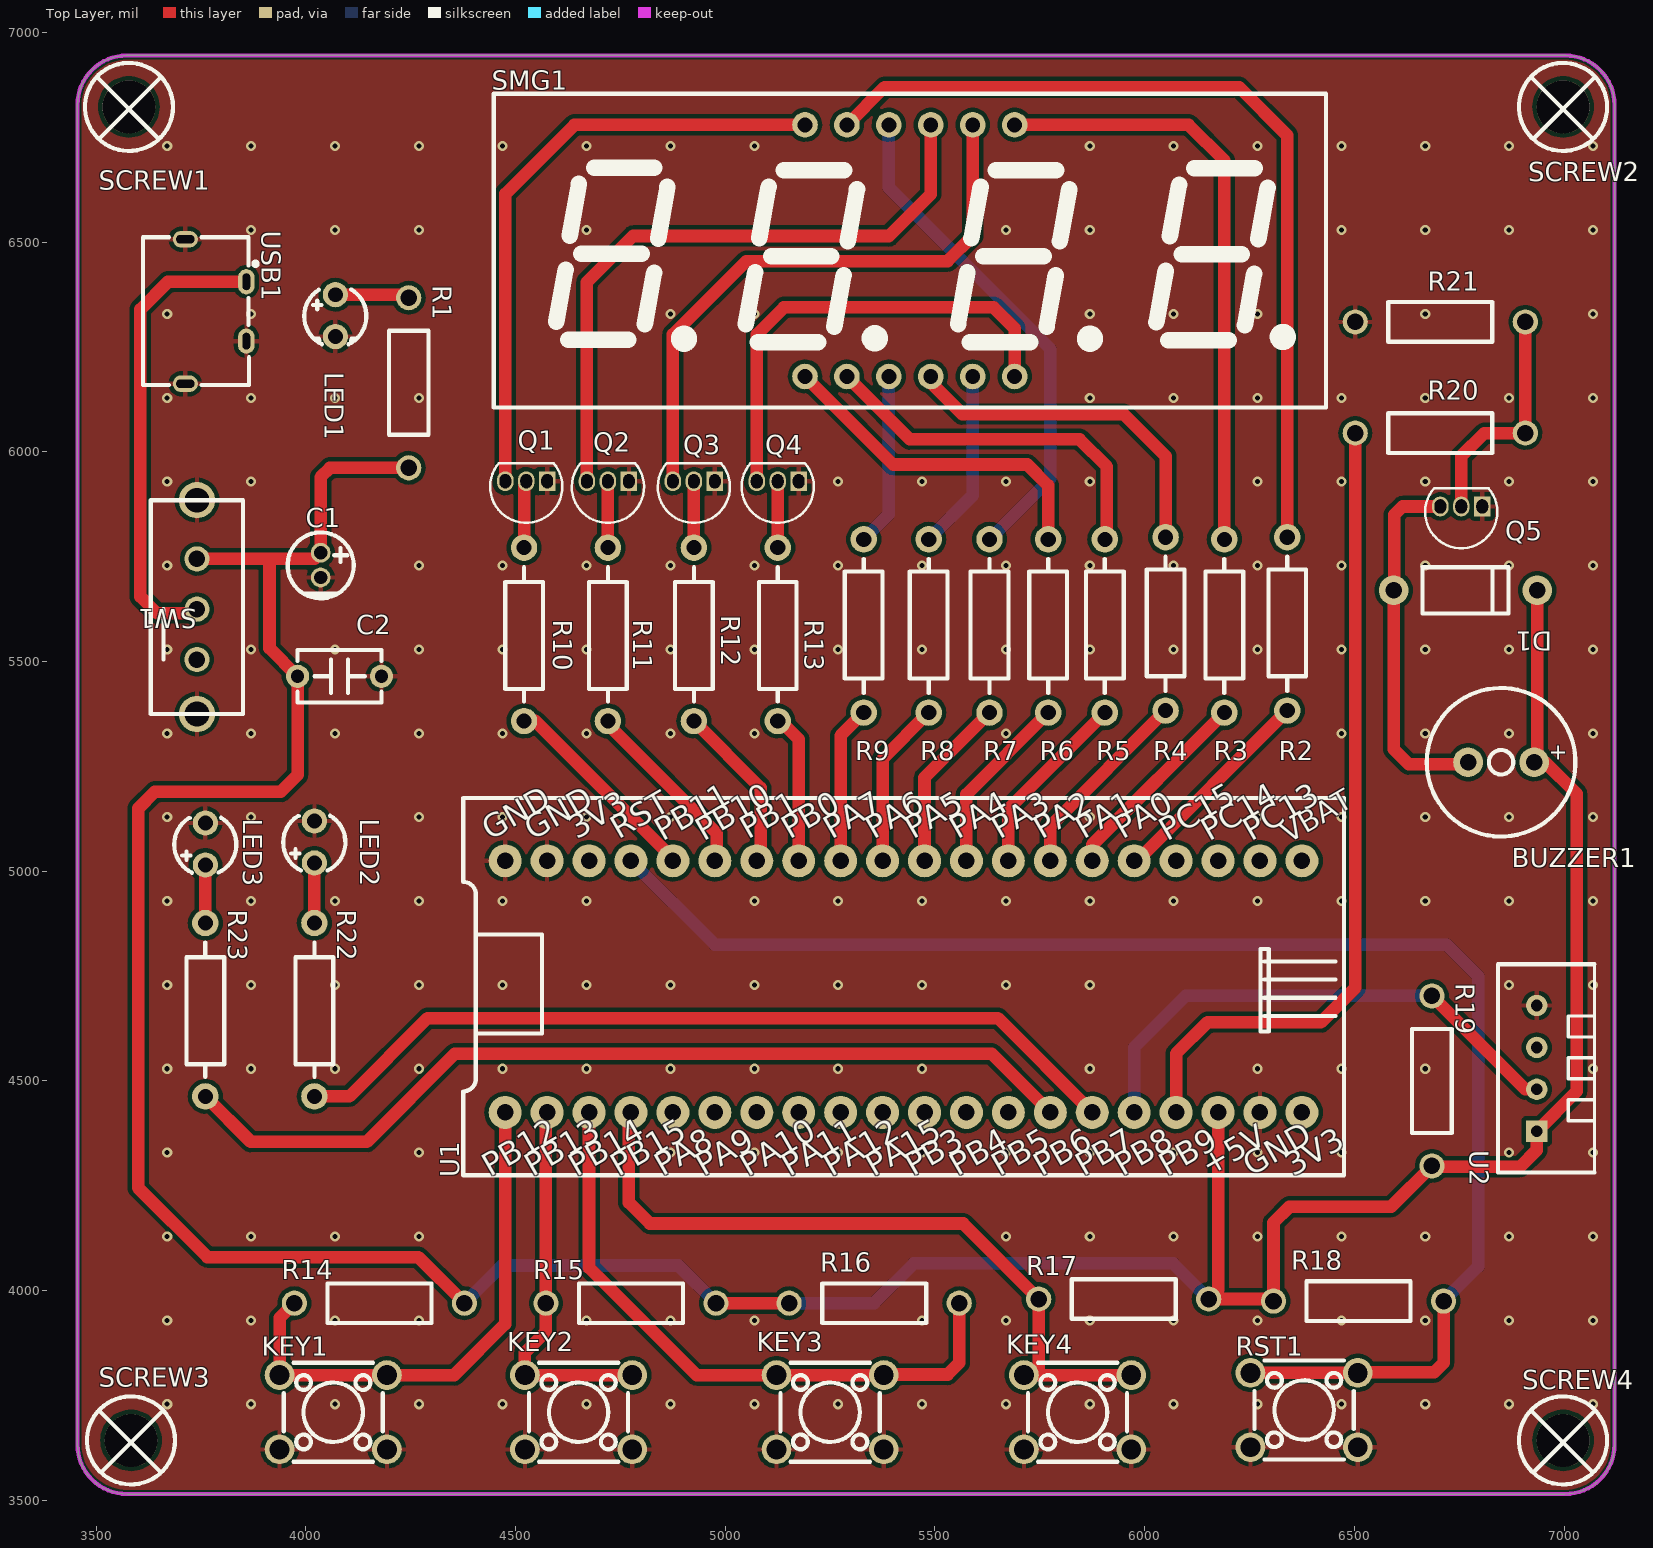
[diagram p0: Top Layer view]
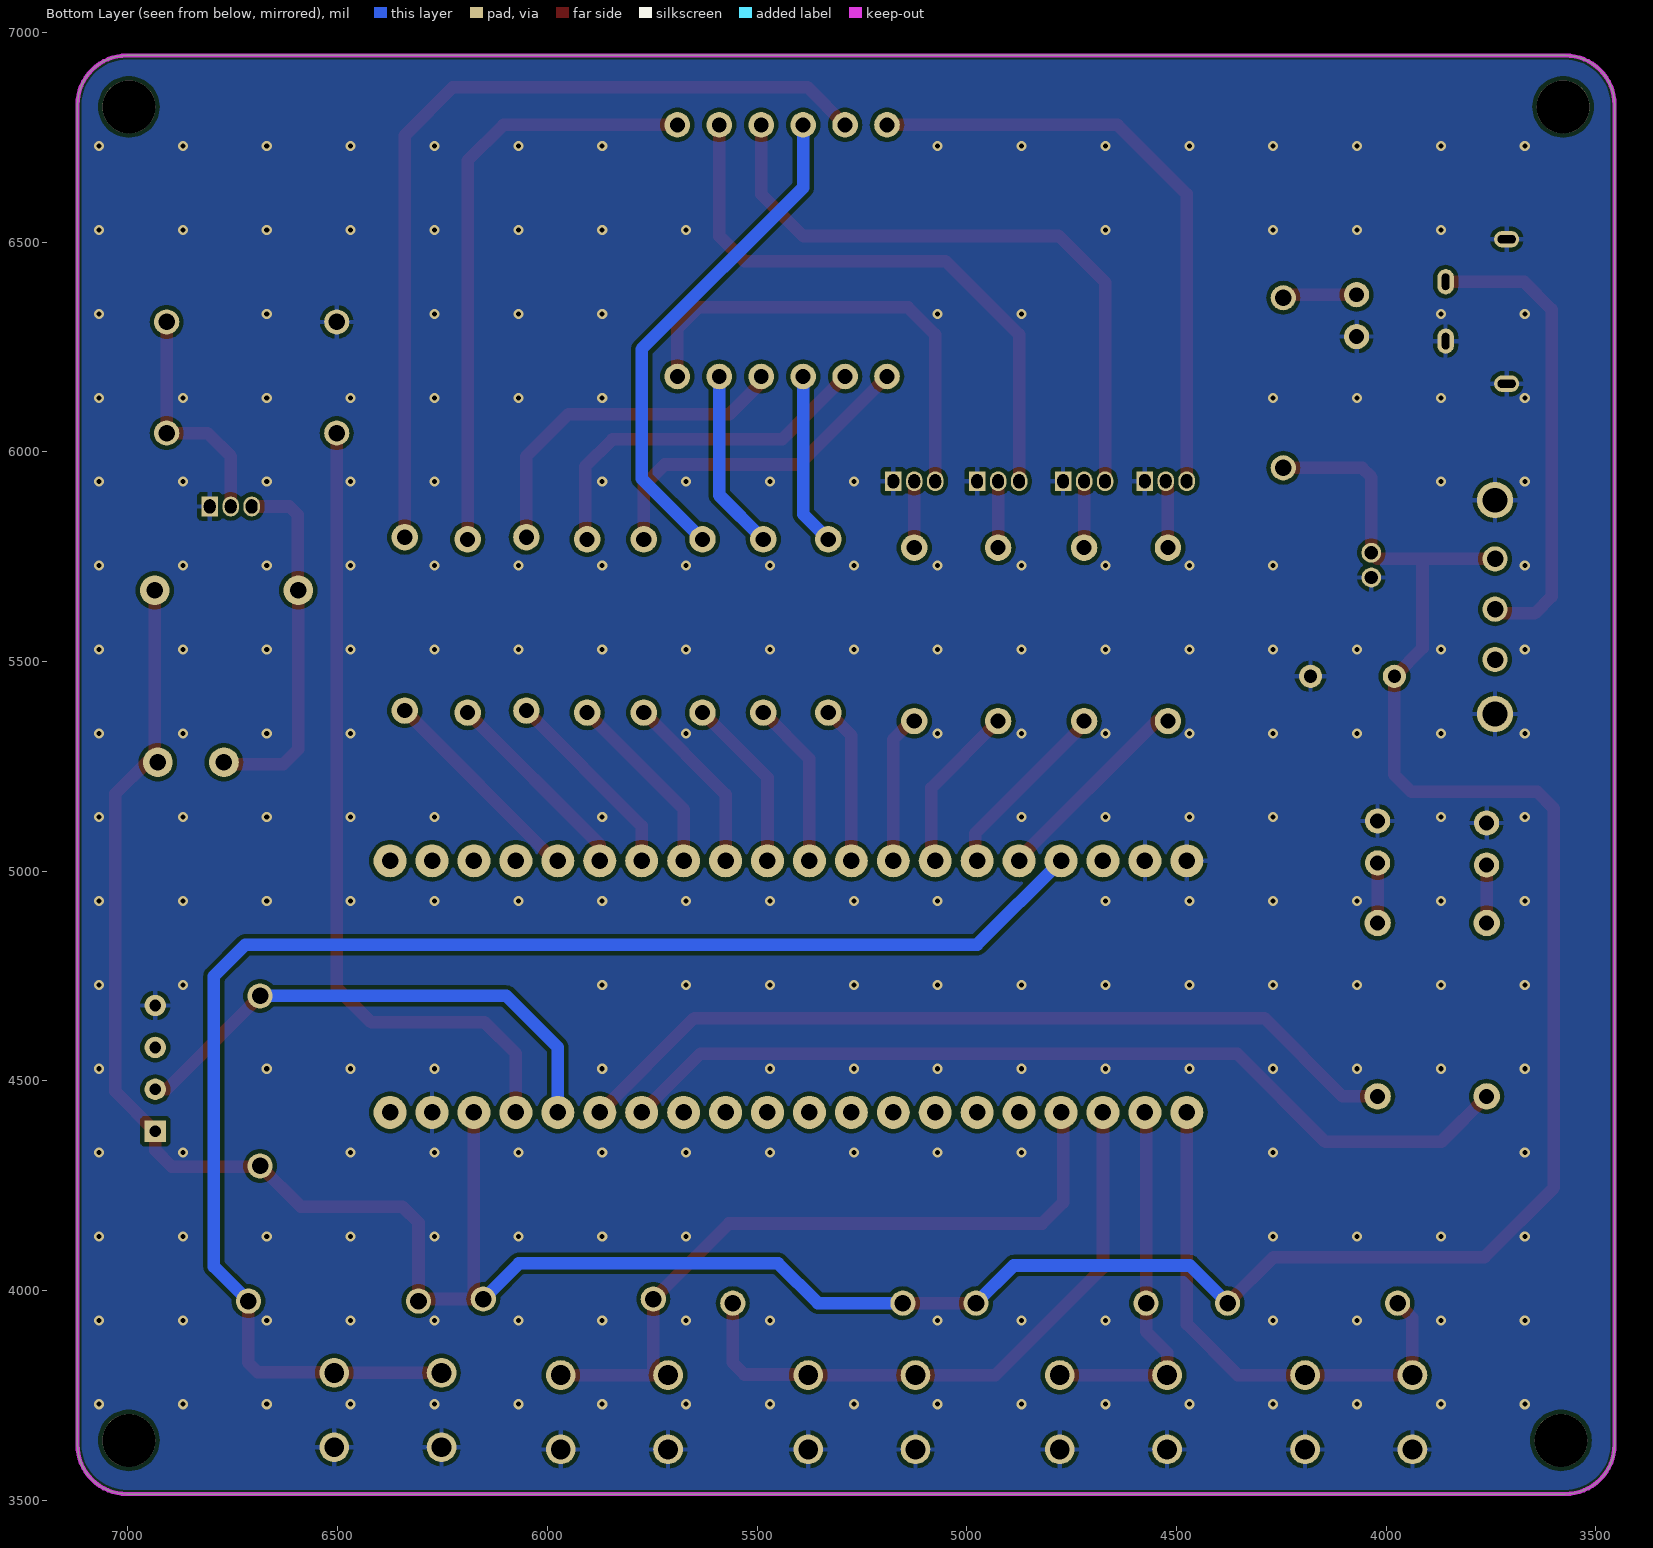
[diagram p1: Bottom Layer view, seen from below]
# Altium PCB MISC61551.pcbdoc
Units mil, origin at the board's own origin, x right, y up, seen from the top; angles counter-clockwise.
Board outline 3665.55 x 3430.55 mil, 2 copper layers (Top Layer, Bottom Layer), stack 62.206 mil thick; 49 components, 45 nets, 164 pads, 222 vias.

## Layer stack, top to bottom
Top Solder Mask Layer: solder mask 0.394, Dk 3.3
Top Layer: signal copper 1.379
Dielectric1: surface 59.449, FR4, Dk 4.5
Bottom Layer: signal copper 1.378
Bottom Solder Mask Layer: solder mask 0.394, Dk 3.3

## Board outline
3573.11,6945.55 ccw(c3573.11,6827.44) 3455,6827.44 3455,3633.11 ccw(c3573.11,3633.11) 3573.11,3515 7002.44,3515 ccw(c7002.44,3633.11) 7120.55,3633.11 7120.55,6827.44 ccw(c7002.44,6827.44) 7002.44,6945.55 3573.11,6945.55

## Design rules (kind name [scope] priority, off if disabled: settings)
BoardOutlineClearance copperThickness2oz_1 [All] p2 off: genericclearance=7.99 ignorepadtopadclearanceinfootprint=FALSE except(0: Arc-SplitContinuation Track-SplitContinuation SMDPad-SplitContinuation THPad-SplitContinuation Via-SplitContinuation Fill-SplitContinuation Region-SplitContinuation Poly-SplitContinuation Text-SplitContinuation Hole-SplitContinuation; 5.98: Arc-CutoutEdge SMDPad-CutoutEdge THPad-CutoutEdge Via-CutoutEdge Fill-CutoutEdge Region-CutoutEdge Text-CutoutEdge; 6.93: Hole-OutlineEdge Hole-CutoutEdge; 10: Poly-OutlineEdge Poly-CutoutEdge; 11.81: Arc-OutlineEdge Track-OutlineEdge SMDPad-OutlineEdge THPad-OutlineEdge Via-OutlineEdge Fill-OutlineEdge Region-OutlineEdge Text-OutlineEdge Track-CutoutEdge)
BoardOutlineClearance copperThickness1oz_1 [All] p4: genericclearance=6 ignorepadtopadclearanceinfootprint=FALSE except(0: Arc-SplitContinuation Track-SplitContinuation SMDPad-SplitContinuation THPad-SplitContinuation Via-SplitContinuation Fill-SplitContinuation Region-SplitContinuation Poly-SplitContinuation Text-SplitContinuation Hole-SplitContinuation; 6: SMDPad-CutoutEdge THPad-CutoutEdge Via-CutoutEdge Fill-CutoutEdge Region-CutoutEdge Text-CutoutEdge; 6.93: Hole-OutlineEdge Hole-CutoutEdge; 10: Poly-OutlineEdge Poly-CutoutEdge; 11.8: Arc-OutlineEdge Track-OutlineEdge SMDPad-OutlineEdge THPad-OutlineEdge Via-OutlineEdge Fill-OutlineEdge Region-OutlineEdge Text-OutlineEdge; 11.81: Arc-CutoutEdge Track-CutoutEdge)
Clearance copperThickness2oz [All] p1 off: gap=7.99 ignorepadtopadclearanceinfootprint=FALSE except(5.98: SMDPad-Track SMDPad-SMDPad THPad-Track SMDPad-THPad THPad-THPad Track-Via SMDPad-Via THPad-Via Via-Via Fill-Track Region-Track Fill-SMDPad Region-SMDPad Fill-THPad Region-THPad Fill-Via Region-Via Fill-Fill Fill-Region Region-Region Arc-Track Arc-SMDPad Arc-THPad Arc-Via Fill-Arc Region-Arc Arc-Arc Text-Track SMDPad-Text Text-THPad Text-Via Fill-Text Region-Text Arc-Text Text-Text; 6.93: Hole-Track Hole-SMDPad Hole-THPad Hole-Via Fill-Hole Region-Hole Hole-Arc Hole-Text; 10: Poly-Track Poly-SMDPad Poly-THPad Poly-Via Poly-Fill Poly-Region Poly-Poly Poly-Arc Poly-Text Poly-Hole)
Clearance copperThickness1oz [All] p3: gap=6 ignorepadtopadclearanceinfootprint=FALSE except(5.98: SMDPad-Track SMDPad-SMDPad THPad-Track SMDPad-THPad THPad-THPad Track-Via SMDPad-Via THPad-Via Via-Via Fill-Track Region-Track Fill-SMDPad Region-SMDPad Fill-THPad Region-THPad Fill-Via Region-Via Fill-Fill Fill-Region Region-Region; 6.93: Hole-Track Hole-SMDPad Hole-THPad Hole-Via Fill-Hole Region-Hole Hole-Arc Hole-Text; 10: Poly-Track Poly-SMDPad Poly-THPad Poly-Via Poly-Fill Poly-Region Poly-Poly Poly-Arc Poly-Text Poly-Hole)
DiffPairsRouting differentialPair [All] p1: maxlimit=6 minlimit=6 mostfreqgap=6 toplayer_minwidth=5 toplayer_prefwidth=10 toplayer_maxwidth=100 toplayer_mingap=6 toplayer_prefgap=6 toplayer_maxgap=6 bottomlayer_minwidth=5 bottomlayer_prefwidth=10 bottomlayer_maxwidth=100 bottomlayer_mingap=6 bottomlayer_prefgap=6 bottomlayer_maxgap=6 maxuncoupledlength=10
HoleToHoleClearance otherClearance [All] p1: gap=11.81 allowstackedmicrovias=TRUE
Length netLength [All] p1: minlimit=0 maxlimit=0
MatchedLengths netLengthTolerance [All] p1: tolerance=1000
PasteMaskExpansion pasteMaskExpansion [All] p1: expansion=0
PlaneConnect innerPlane [All] p1: planeconnectstyle=Relief reliefexpansion=20 reliefentries=4 reliefconductorwidth=10 reliefairgap=10
PolygonConnect copperRegion [(InNet('GND'))] p1: connectstyle=Relief reliefconductorwidth=10 reliefentries=4 polygonreliefangle="90 Angle" airgapwidth=10 via.connectstyle=Relief via.reliefconductorwidth=10 via.reliefentries=4 via.polygonreliefangle="90 Angle" via.airgapwidth=10
RoutingVias viaSize [All] p1: holewidth=12.01 width=24.02 viastyle="Through Hole" minholewidth=12 minwidth=24 maxholewidth=248.03 maxwidth=393.7
SolderMaskExpansion solderMaskExpansion [IsVia] p1: expansion=-1000 istentingtop=TRUE
SolderMaskExpansion solderMaskExpansion [All] p2: expansion=2 istentingtop=FALSE
Width copperThickness2oz_2 [All] p1 off: maxlimit=100 minlimit=8 preferedwidth=10
Width PWR [(InNet('+5V') OR InNet('BUZZER') OR InNet('DIG1') OR InNet('DIG2') OR InNet('DIG3') OR InNet('DIG4') OR InNet('VCC'))] p2: maxlimit=10 minlimit=10 preferedwidth=10 toplayer_minwidth=10 toplayer_maxwidth=100 toplayer_prefwidth=20 bottomlayer_minwidth=10 bottomlayer_maxwidth=100 bottomlayer_prefwidth=20
Width copperThickness1oz_2 [All] p3: maxlimit=10 minlimit=10 preferedwidth=10 toplayer_minwidth=10 toplayer_maxwidth=100 toplayer_prefwidth=10 bottomlayer_minwidth=10 bottomlayer_maxwidth=100 bottomlayer_prefwidth=10

## Components (designator, comment, footprint, x,y, rotation, side; value= is the part's Value field where it differs from the comment)
BUZZER1 "2.7kHz" BUZ-TH_BD9.0-P4.00-D0.6-FD 6850,5260 r180 top
C1 "10uF" CAP-TH_BD4.0-P1.50-D0.8-FD 4035,5730 r270 top
C2 "100nF" CAP-TH_L5.0-W2.5-P5.08-D0.7 4080,5465 r180 top
D1 "1N5819" DO-41_BD2.4-L4.7-P8.70-D0.9-RD 6765,5670 r180 top
KEY1 "TS-1002-07026" SW-TH_4P-L6.0-W6.0-P4.50-LS6.5 4065,3710 r0 top
KEY2 "TS-1002-07026" SW-TH_4P-L6.0-W6.0-P4.50-LS6.5 4650,3710 r0 top
KEY3 "TS-1002-07026" SW-TH_4P-L6.0-W6.0-P4.50-LS6.5 5250,3710 r0 top
KEY4 "TS-1002-07026" SW-TH_4P-L6.0-W6.0-P4.50-LS6.5 5840,3710 r0 top
LED1 "XL-302SURD" LED-TH_BD3.8-P2.54-RD 4070,6325 r90 top
LED2 "XL-302UGD" LED-TH_BD3.8-P2.54-FD_GREEN 4020,5070 r90 top
LED3 "XL-302UGD" LED-TH_BD3.8-P2.54-FD_GREEN 3760,5065 r90 top
Q1 "S8050" TO-92-3_L4.5-W3.5-P1.27-L 4525.27,5930.27 r180 top
Q2 "S8050" TO-92-3_L4.5-W3.5-P1.27-L 4720,5930 r180 top
Q3 "S8050" TO-92-3_L4.5-W3.5-P1.27-L 4925,5930 r180 top
Q4 "S8050" TO-92-3_L4.5-W3.5-P1.27-L 5125,5930 r180 top
Q5 "S8050" TO-92-3_L4.5-W3.5-P1.27-L 6755,5870 r180 top
R1 "10kΩ" RES-TH_BD2.4-L6.3-P10.30-D0.6 4245,6165 r270 top
R2 "330Ω" RES-TH_BD2.2-L6.5-P10.50-D0.6 6340,5590 r90 top
R3 "330Ω" RES-TH_BD2.2-L6.5-P10.50-D0.6 6190,5585 r90 top
R4 "330Ω" RES-TH_BD2.2-L6.5-P10.50-D0.6 6050,5590 r90 top
R5 "330Ω" RES-TH_BD2.2-L6.5-P10.50-D0.6 5905,5585 r90 top
R6 "330Ω" RES-TH_BD2.2-L6.5-P10.50-D0.6 5770,5585 r90 top
R7 "330Ω" RES-TH_BD2.2-L6.5-P10.50-D0.6 5630,5585 r90 top
R8 "330Ω" RES-TH_BD2.2-L6.5-P10.50-D0.6 5485,5585 r90 top
R9 "330Ω" RES-TH_BD2.2-L6.5-P10.50-D0.6 5330,5585 r90 top
R10 "1kΩ" RES-TH_BD2.2-L6.5-P10.50-D0.6 4520,5565 r270 top
R11 "1kΩ" RES-TH_BD2.2-L6.5-P10.50-D0.6 4720,5565 r270 top
R12 "1kΩ" RES-TH_BD2.2-L6.5-P10.50-D0.6 4925,5565 r270 top
R13 "1kΩ" RES-TH_BD2.2-L6.5-P10.50-D0.6 5125,5565 r270 top
R14 "10kΩ" RES-TH_BD2.4-L6.3-P10.30-D0.6 4175,3970 r0 top
R15 "10kΩ" RES-TH_BD2.4-L6.3-P10.30-D0.6 4775,3970 r0 top
R16 "10kΩ" RES-TH_BD2.4-L6.3-P10.30-D0.6 5355,3970 r180 top
R17 "10kΩ" RES-TH_BD2.4-L6.3-P10.30-D0.6 5950,3980 r0 top
R18 "10kΩ" RES-TH_BD2.4-L6.3-P10.30-D0.6 6510,3975 r180 top
R19 "10kΩ" RES-TH_BD2.4-L6.3-P10.30-D0.6 6685,4500 r270 top
R20 "10kΩ" RES-TH_BD2.4-L6.3-P10.30-D0.6 6705,6045 r180 top
R21 "10kΩ" RES-TH_BD2.4-L6.3-P10.30-D0.6 6705,6310 r0 top
R22 "1kΩ" RES-TH_BD2.2-L6.5-P10.50-D0.6 4020,4670 r270 top
R23 "1kΩ" RES-TH_BD2.2-L6.5-P10.50-D0.6 3760,4670 r270 top
RST1 "TS-1002-07026" SW-TH_4P-L6.0-W6.0-P4.50-LS6.5 6380.27,3715.27 r0 top
SCREW1 "" M3螺丝 3580.27,6820.27 r0 top locked
SCREW2 "" M3螺丝 7000.27,6820.27 r0 top locked
SCREW3 "" M3螺丝 3585.27,3640.27 r0 top locked
SCREW4 "" M3螺丝 7000.27,3640.27 r0 top locked
SMG1 "" LED-SEG-TH_FJ5461AH 5440,6480 r0 top
SW1 "SK-12E12-G5" SW-TH_SK-12E12-G5 3740,5630 r180 top
U1 "" GD32E230C8T6最小系统 4475,4425 r90 top
U2 "DHT11" SENSOR-TH_DHT11 6935,4530 r90 top
USB1 "KH-TYPE-C-2P" USB-SMD_KH-TYPE-C-2P 3785,6335 r270 top

## Footprints (in the part's own frame and the unit in brackets; to place one, negate y for a bottom-side part, rotate by r counter-clockwise, add the part's x,y. Pads: shape width x height; smd on the part's side, far side on the other; paste and mask are expansions set on the pad)
BUZ-TH_BD9.0-P4.00-D0.6-FD [mm]
  round 1.8 hole 1: 1(-2,0) 2(2,0)
  silkscreen extent -4.5,-4.5 4.5,4.5
CAP-TH_BD4.0-P1.50-D0.8-FD [mm]
  round 1.2 hole 0.8: 1(-0.75,0) 2(0.75,0)
  silkscreen extent -1.98,-2 2.06,2
CAP-TH_L5.0-W2.5-P5.08-D0.7 [mm]
  round 1.4 hole 0.8: 1(-2.54,0) 2(2.54,0)
  silkscreen extent -2.54,-1.59 2.54,1.59
DO-41_BD2.4-L4.7-P8.70-D0.9-RD [mm]
  round 1.8 hole 1: 1(-4.35,0) 2(4.35,0)
  silkscreen extent -2.6,-1.4 2.6,1.4
GD32E230C8T6最小系统 [mm]
  round 2 hole 1: 1(0,0) 2(0,-2.54) 3(0,-5.08) 4(0,-7.62) 5(0,-10.16) 6(0,-12.7) 7(0,-15.24) 8(0,-17.78) 9(0,-20.32) 10(0,-22.86) 11(0,-25.4) 12(0,-27.94) 13(0,-30.48) 14(0,-33.02) 15(0,-35.56) 16(0,-38.1) 17(0,-40.64) 18(0,-43.18) 19(0,-45.72) 20(0,-48.26) 21(15.24,-48.26) 22(15.24,-45.72) 23(15.24,-43.18) 24(15.24,-40.64) 25(15.24,-38.1) 26(15.24,-35.56) 27(15.24,-33.02) 28(15.24,-30.48) 29(15.24,-27.94) 30(15.24,-25.4) 31(15.24,-22.86) 32(15.24,-20.32) 33(15.24,-17.78) 34(15.24,-15.24) 35(15.24,-12.7) 36(15.24,-10.16) 37(15.24,-7.62) 38(15.24,-5.08) 39(15.24,-2.54) 40(15.24,0)
  silkscreen extent -3.81,-50.8 19.05,2.54
LED-SEG-TH_FJ5461AH [mm]
  round 1.55 hole 0.9: 1(-6.35,-7.62) 2(-3.81,-7.62) 3(-1.27,-7.62) 4(1.27,-7.62) 5(3.81,-7.62) 6(6.35,-7.62) 7(6.35,7.62) 8(3.81,7.62) 9(1.27,7.62) 10(-1.27,7.62) 11(-3.81,7.62) 12(-6.35,7.62)
  silkscreen extent -25.2,-9.5 25.2,9.5
LED-TH_BD3.8-P2.54-FD_GREEN [mil]
  round 60 hole 35.43: 1(-50,0) 2(50,0)
  silkscreen extent -68,-74 63,74
LED-TH_BD3.8-P2.54-RD [mil]
  round 60 hole 35.43: 1(-50,0) 2(50,0)
  silkscreen extent -68,-74 63,74
M3螺丝 [mil]
  round 126 hole 126 paste+0 mask+4: 1(-2.5,2.5)
  silkscreen extent -107,-102 102,107
RES-TH_BD2.2-L6.5-P10.50-D0.6 [mm]
  round 1.6 hole 0.914: 1(-5.25,0) 2(5.25,0)
  silkscreen extent -4.06,-1.14 4.06,1.14
RES-TH_BD2.4-L6.3-P10.30-D0.6 [mil]
  round 60 hole 39.37: 1(-202.76,0) 2(202.76,0)
  silkscreen extent -124,-47 124,47
SENSOR-TH_DHT11 [mil]
  rect 51x51 hole 28: 1(-150,0)
  round 51 hole 28: 2(-50,0) 3(50,0) 4(150,0)
  silkscreen extent -248,-138 248,93
SW-TH_4P-L6.0-W6.0-P4.50-LS6.5 [mm]
  round 1.8 hole 1.2: 1(-3.25,2.25) 2(3.25,2.25) 3(-3.25,-2.25) 4(3.25,-2.25)
  silkscreen extent -3,-3 3,3
SW-TH_SK-12E12-G5 [mil]
  round 60 hole 39.37: 1(0,125) 2(0,5) 3(0,-115)
  round 86.61 hole 59.06: 4(0,-255) 5(0,255)
  silkscreen extent -110,-255 110,255
TO-92-3_L4.5-W3.5-P1.27-L [mm]
  rect 1x1.2 hole 0.7 slot 0.85 at 90 deg: 1(-1.27,0)
  oval 1x1.2 hole 0.7 slot 0.85 at 90 deg: 2(0,0) 3(1.27,0)
  silkscreen extent -2.19,-1.1 2.19,2.52
USB-SMD_KH-TYPE-C-2P [mm]
  oval 1.524x1 hole 0.45 slot 1 at 0 deg paste+0 mask+0.05: 1(-1.8,1.85) 2(1.8,1.85)
  oval 1x1.524 hole 0.5 slot 1.1 at 90 deg paste+0 mask+0.05: 3(4.375,-1.85) 4(-4.375,-1.85)
  silkscreen extent -4.5,-4.41 4.46,2.53

## Via types
v1: diameter 24.02, hole 12, Top Layer to Bottom Layer, 222 vias

## Nets (pads, with @x,y where several pads share a name; then routed paths per layer and width w, separated by ;. In a path a pad name is that pad's centre, name@x,y a point inside that pad or via, vN(x,y) a via of type N, cw(c..) or ccw(c..) an arc to the next point about the centre after c; other vN are vias at no path point)
$1N759: BUZZER1.2 D1.2 Q5.3 | length 872.2
  Top Layer w30: Q5.3 6615,5870 6595,5850 6595,5671.26 D1.2 6593.74,5291.26 6630,5255 6766.26,5255 BUZZER1.2
$1N845: Q5.2 R20.1 R21.2 | length 560.5
  Top Layer w30: Q5.2 6755,5990 6810,6045 R20.1 R21.2
$1N1452: LED3.1 R23.1 | length 138.3
  Top Layer w30: R23.1 LED3.1
$1N1457: LED2.1 R22.1 | length 143.3
  Top Layer w30: R22.1 LED2.1
$1N2594: LED1.2 R1.1 | length 178
  Top Layer w30: LED1.2 4237.76,6375 R1.1
$1N4493: Q1.3 SMG1.12 | length 1468
  Top Layer w30: Q1.3 4475.27,6615.27 4640,6780 SMG1.12
$1N5128: R2.2 SMG1.11 | length 2093.2
  Top Layer w30: SMG1.11 5380,6870 6225,6870 6340,6755 R2.2
$1N5138: R9.2 SMG1.3 | length 413.2
  Bottom Layer w30: R9.2 5390,5851.69 SMG1.3
$1N5143: R8.2 SMG1.5 | length 431.8
  Bottom Layer w30: R8.2 5590,5896.69 SMG1.5
$1N5148: R3.2 SMG1.7 | length 1438.5
  Top Layer w30: SMG1.7 6105,6780 6190,6695 R3.2
$1N5153: R4.2 SMG1.4 | length 840.8
  Top Layer w30: SMG1.4 5490,6165 5565,6090 5950,6090 6050,5990 R4.2
$1N5158: R5.2 SMG1.2 | length 884.4
  Top Layer w30: SMG1.2 5440,6030 5845,6030 5910,5965 5910,5796.69 R5.2
$1N5162: R6.2 SMG1.1 | length 816
  Top Layer w30: SMG1.1 5400,5970 5720,5970 5770,5920 R6.2
$1N5166: R7.2 SMG1.10 | length 1207.8
  Bottom Layer w30: SMG1.10 5390,6630 5775,6245 5775,5936.69 R7.2
$1N5201: Q1.2 R10.1 | length 160.8
  Top Layer w30: R10.1 4520,5925 Q1.2
$1N5302: Q2.2 R11.1 | length 158.3
  Top Layer w30: R11.1 Q2.2
$1N5397: Q3.2 R12.1 | length 158.3
  Top Layer w30: R12.1 Q3.2
$1N5492: Q4.2 R13.1 | length 158.3
  Top Layer w30: R13.1 Q4.2
$1N5499: Q2.3 SMG1.9 | length 1547
  Top Layer w30: Q2.3 4670,6405 4780,6515 5390,6515 5490,6615 SMG1.9
$1N5503: Q3.3 SMG1.8 | length 1427.3
  Top Layer w30: Q3.3 4875,6280 5050,6455 5530,6455 5590,6515 SMG1.8
$1N5507: Q4.3 SMG1.6 | length 1127.6
  Top Layer w30: Q4.3 5075,6280 5140,6345 5640,6345 5690,6295 SMG1.6
+5V: BUZZER1.1 C1.1 C2.2 D1.1 R1.2 R14.2 R15.2 R16.2 R17.2 R18.2 R19.2 SW1.3 U1.18 U2.1 | length 8311.4
  Top Layer w30: SW1.3 3912.94,5745 ; R1.2 4057.24,5962.24 4035,5940 C1.1 4020.47,5745 3912.94,5745 ; R14.2 4267.76,4080 3765,4080 3600,4245 3600,5150 3640,5190 3940,5190 3980,5230 C2.2 3912.94,5532.06 3912.94,5745 ; R15.2 R16.2 ; U1.18 6175,4002.24 R17.2 6302.24,3980 R18.2 6307.24,4162.24 6345,4200 6587.76,4200 R19.2 6687.24,4295 6895,4295 6935,4335 U2.1 7030,4475 7030,5185 6955,5260 BUZZER1.1 6936.26,5267.52 D1.1
  Bottom Layer w30: R14.2 4467.76,4060 4887.76,4060 R15.2 ; R16.2 5355,3970 5450,4065 6067.76,4065 R17.2
BUZZER: R20.2 U1.17 | length 1955.1
  Top Layer w30: U1.17 6075,4565 6150,4640 6420,4640 6502.24,4722.24 R20.2
DHT11: R19.1 U1.16 U2.2 | length 1258.1
  Top Layer w30: R19.1 6907.76,4480 U2.2
  Bottom Layer w30: U1.16 5975,4580 6097.76,4702.76 R19.1
DIG1: R10.2 U1.36 | length 496
  Top Layer w30: R10.2 4546.69,5358.31 4875,5030 U1.36
DIG2: R11.2 U1.35 | length 443.1
  Top Layer w30: R11.2 4720,5350 4980,5090 4980,5030 U1.35
DIG3: R12.2 U1.34 | length 403
  Top Layer w30: R12.2 5084.14,5199.16 5084.14,5034.14 U1.34
DIG4: R13.2 U1.33 | length 357.9
  Top Layer w30: R13.2 5131.69,5358.31 5175,5315 U1.33
GND: C1.2 C2.1 KEY1.3 KEY1.4 KEY2.3 KEY2.4 KEY3.3 KEY3.4 KEY4.3 KEY4.4 LED1.1 LED2.2 LED3.2 Q1.1 Q2.1 Q3.1 Q4.1 Q5.1 R21.1 RST1.3 RST1.4 SW1.4 SW1.5 U1.19 U1.39 U1.40 U2.4 USB1.2 USB1.3 USB1.4
  other v1: 3669.1,3729.1 3869.1,3729.1 4069.1,3729.1 4269.1,3729.1 4469.1,3729.1 4669.1,3729.1 4869.1,3729.1 5069.1,3729.1 5269.1,3729.1 5469.1,3729.1 5669.1,3729.1 5869.1,3729.1 6069.1,3729.1 6269.1,3729.1 6469.1,3729.1 6669.1,3729.1 6869.1,3729.1 7069.1,3729.1 3669.1,3929.1 3869.1,3929.1 4069.1,3929.1 4269.1,3929.1 4669.1,3929.1 4869.1,3929.1 5069.1,3929.1 5469.1,3929.1 5669.1,3929.1 5869.1,3929.1 6069.1,3929.1 6269.1,3929.1 6469.1,3929.1 6669.1,3929.1 6869.1,3929.1 7069.1,3929.1 3669.1,4129.1 3869.1,4129.1 4069.1,4129.1 4269.1,4129.1 5669.1,4129.1 5869.1,4129.1 6069.1,4129.1 6269.1,4129.1 6469.1,4129.1 6669.1,4129.1 6869.1,4129.1 7069.1,4129.1 3669.1,4329.1 4269.1,4329.1 4869.1,4329.1 5069.1,4329.1 5269.1,4329.1 5469.1,4329.1 5669.1,4329.1 5869.1,4329.1 6069.1,4329.1 6269.1,4329.1 6469.1,4329.1 6869.1,4329.1 7069.1,4329.1 3669.1,4529.1 3869.1,4529.1 4069.1,4529.1 4269.1,4529.1 4469.1,4529.1 4669.1,4529.1 4869.1,4529.1 5069.1,4529.1 5269.1,4529.1 5469.1,4529.1 5869.1,4529.1 6269.1,4529.1 6469.1,4529.1 6669.1,4529.1 7069.1,4529.1 3669.1,4729.1 3869.1,4729.1 4069.1,4729.1 4269.1,4729.1 4469.1,4729.1 4669.1,4729.1 4869.1,4729.1 5069.1,4729.1 5269.1,4729.1 5469.1,4729.1 5669.1,4729.1 5869.1,4729.1 6869.1,4729.1 7069.1,4729.1 3669.1,4929.1 3869.1,4929.1 4069.1,4929.1 4269.1,4929.1 4469.1,4929.1 4669.1,4929.1 5069.1,4929.1 5269.1,4929.1 5469.1,4929.1 5669.1,4929.1 5869.1,4929.1 6069.1,4929.1 6269.1,4929.1 6469.1,4929.1 6669.1,4929.1 6869.1,4929.1 7069.1,4929.1 3669.1,5129.1 3869.1,5129.1 4269.1,5129.1 4469.1,5129.1 4669.1,5129.1 4869.1,5129.1 5869.1,5129.1 6269.1,5129.1 6469.1,5129.1 6669.1,5129.1 6869.1,5129.1 7069.1,5129.1 3669.1,5329.1 3869.1,5329.1 4069.1,5329.1 4269.1,5329.1 4469.1,5329.1 4669.1,5329.1 4869.1,5329.1 5069.1,5329.1 5669.1,5329.1 6469.1,5329.1 6669.1,5329.1 6869.1,5329.1 7069.1,5329.1 3669.1,5529.1 3869.1,5529.1 4069.1,5529.1 4269.1,5529.1 4469.1,5529.1 4669.1,5529.1 4869.1,5529.1 5069.1,5529.1 5269.1,5529.1 5469.1,5529.1 5669.1,5529.1 5869.1,5529.1 6069.1,5529.1 6269.1,5529.1 6469.1,5529.1 6669.1,5529.1 6869.1,5529.1 7069.1,5529.1 3669.1,5729.1 4269.1,5729.1 4469.1,5729.1 4669.1,5729.1 4869.1,5729.1 5069.1,5729.1 5269.1,5729.1 5469.1,5729.1 5669.1,5729.1 5869.1,5729.1 6069.1,5729.1 6269.1,5729.1 6469.1,5729.1 6669.1,5729.1 6869.1,5729.1 7069.1,5729.1 3669.1,5929.1 3869.1,5929.1 5269.1,5929.1 5469.1,5929.1 5669.1,5929.1 5869.1,5929.1 6269.1,5929.1 6469.1,5929.1 6669.1,5929.1 6869.1,5929.1 7069.1,5929.1 3669.1,6129.1 3869.1,6129.1 4069.1,6129.1 4269.1,6129.1 5869.1,6129.1 6069.1,6129.1 6269.1,6129.1 6469.1,6129.1 6669.1,6129.1 6869.1,6129.1 7069.1,6129.1 3669.1,6329.1 3869.1,6329.1 4869.1,6329.1 5069.1,6329.1 5869.1,6329.1 6069.1,6329.1 6269.1,6329.1 6669.1,6329.1 7069.1,6329.1 3869.1,6529.1 4069.1,6529.1 4269.1,6529.1 4669.1,6529.1 5669.1,6529.1 5869.1,6529.1 6069.1,6529.1 6269.1,6529.1 6469.1,6529.1 6669.1,6529.1 6869.1,6529.1 7069.1,6529.1 3669.1,6729.1 3869.1,6729.1 4069.1,6729.1 4269.1,6729.1 4469.1,6729.1 4669.1,6729.1 4869.1,6729.1 5069.1,6729.1 5869.1,6729.1 6069.1,6729.1 6269.1,6729.1 6469.1,6729.1 6669.1,6729.1 6869.1,6729.1 7069.1,6729.1
KEY1-PB12: KEY1.1 KEY1.2 R14.1 U1.1 | length 1279.2
  Top Layer w30: R14.1 3937.05,3934.81 KEY1.1 KEY1.2 4353.58,3798.58 4475,3920 U1.1
KEY2-PB13: KEY2.1 KEY2.2 R15.1 U1.2 | length 904.3
  Top Layer w30: U1.2 4572.24,4422.24 R15.1 4572.24,3902.24 4522.05,3852.05 KEY2.1 KEY2.2
KEY3-PB14: KEY3.1 KEY3.2 R16.1 U1.3 | length 1513.3
  Top Layer w30: U1.3 4675,4055 4931.42,3798.58 KEY3.1 KEY3.2 5379.37,3800 5530,3800 5557.76,3827.76 R16.1
KEY4-PB15: KEY4.1 KEY4.2 R17.1 U1.4 | length 1727.2
  Top Layer w30: U1.4 4770,4420 4770,4210 4820,4160 5567.24,4160 R17.1 5747.24,3799.22 5747.88,3798.58 ; KEY4.1 5747.88,3798.58 ; KEY4.2 5747.88,3798.58
LED1: R23.2 U1.14 | length 2204.8
  Top Layer w30: R23.2 3868.3,4355 4145,4355 4355,4565 5635,4565 U1.14
LED2: R22.2 U1.15 | length 2025.5
  Top Layer w30: R22.2 4103.31,4463.31 4290,4650 5650,4650 U1.15
RST: R18.1 RST1.1 RST1.2 U1.37 | length 3560.6
  Top Layer w30: RST1.1 RST1.2 6509.37,3805 6690,3805 6712.76,3827.76 R18.1
  Bottom Layer w30: U1.37 4975,4825 6720,4825 6795,4750 6795,4057.24 R18.1
SMG_A: R2.1 U1.25 | length 513.4
  Top Layer w30: U1.25 5981.69,5025 R2.1
SMG_B: R3.1 U1.26 | length 483.8
  Top Layer w30: U1.26 5875,5063.31 R3.1
SMG_C: R4.1 U1.27 | length 472.2
  Top Layer w30: U1.27 5775,5108.31 R4.1
SMG_D: R5.1 U1.28 | length 448.6
  Top Layer w30: U1.28 5675,5148.31 R5.1
SMG_DP: R9.1 U1.32 | length 376.1
  Top Layer w30: U1.32 5275,5323.31 R9.1
SMG_E: R6.1 U1.29 | length 434.1
  Top Layer w30: U1.29 5575,5183.31 R6.1
SMG_F: R7.1 U1.30 | length 417.5
  Top Layer w30: U1.30 5475,5223.31 R7.1
SMG_G: R8.1 U1.31 | length 398.9
  Top Layer w30: U1.31 5375,5268.31 R8.1
VCC: SW1.2 USB1.1 | length 1120.8
  Top Layer w30: SW1.2 3730,5615 3645,5615 3605,5655 3605,6340 3670.87,6405.87 USB1.1
pads on no net: SCREW1.1 SCREW2.1 SCREW3.1 SCREW4.1 SW1.1 U1.5 U1.6 U1.7 U1.8 U1.9 U1.10 U1.11 U1.12 U1.13 U1.20 U1.21 U1.22 U1.23 U1.24 U1.38 U2.3

## Polygon pours and split planes (outlines as drawn)
GND on Top Layer (solid, remove dead copper, pour order 0): 3000,7440 3000,3000 7460,3000 7460,7440
GND on Bottom Layer (solid, remove dead copper, pour order 2): 3215,7190 3215,3245 7520,3245 7520,7190

## Keep-outs
Board Outline Layer:
  the board outline again, w10